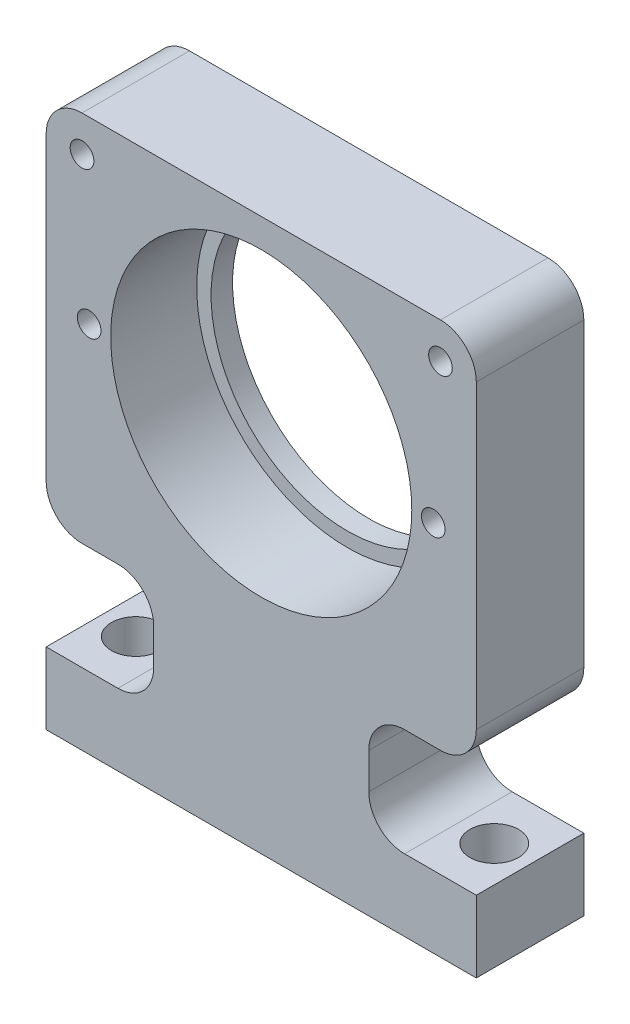
from build123d import *

# Parameters (mm, degrees)
BOSS_EXTRUDE1_DEPTH = 7.5
SKETCH2_R           = 3.4
CUT_EXTRUDE1_DEPTH  = 15
SKETCH4_R           = 19
CUT_EXTRUDE3_DEPTH  = 84.988094394
SKETCH3_R           = 21
CUT_EXTRUDE4_DEPTH  = 12
M4_TAPPED_HOLE2_D   = 3.3
M4_TAPPED_HOLE1_D   = 3.3
FILLET2_R           = 5


with BuildPart() as part:
    # Sketch1 → Boss-Extrude1 (new, symmetric)
    with BuildSketch(Plane.XY):
        Polygon((30, 0), (-30, 0), (-30, 10), (-15, 10), (-15, 25), (-30, 25), (-30, 77), (30, 77), (30, 25), (15, 25), (15, 10), (30, 10), align=None)
    extrude(amount=BOSS_EXTRUDE1_DEPTH, both=True)

    # Sketch2 → Cut-Extrude1 (cut)
    with BuildSketch(Plane.XZ):
        with Locations(Location((-25, 0, 0), (0, 0, 270))):
            Circle(SKETCH2_R)
        with Locations(Location((25, 0, 0), (0, 0, 270))):
            Circle(SKETCH2_R)
    extrude(amount=-CUT_EXTRUDE1_DEPTH, mode=Mode.SUBTRACT)

    # Sketch4 → Cut-Extrude3 (cut, through all)
    with BuildSketch(Plane.XY.offset(7.5)):
        with Locations((0, 52)):
            Circle(SKETCH4_R)
    extrude(amount=-CUT_EXTRUDE3_DEPTH, mode=Mode.SUBTRACT)

    # Sketch3 → Cut-Extrude4 (cut)
    with BuildSketch(Plane.XY.offset(7.5)):
        with Locations((0, 52)):
            Circle(SKETCH3_R)
    extrude(amount=-CUT_EXTRUDE4_DEPTH, mode=Mode.SUBTRACT)

    # M4 Tapped Hole2 (through all)
    with Locations(Plane.XY.offset(7.5)):
        with Locations((24, 52), (-24, 52)):
            Hole(M4_TAPPED_HOLE2_D / 2)

    # M4 Tapped Hole1 (through all)
    with Locations(Plane.XY.offset(7.5)):
        with Locations((-25, 72), (25, 72)):
            Hole(M4_TAPPED_HOLE1_D / 2)

    # Fillet2
    fillet2_edges = [part.edges().sort_by_distance(p)[0] for p in [
        (-30, 25, 0),
        (-30, 77, 0),
        (30, 77, 0),
        (30, 25, 0),
        (15, 25, 0),
        (15, 10, 0),
        (-15, 10, 0),
        (-15, 25, 0),
    ]]
    fillet(fillet2_edges, radius=FILLET2_R)


solid = part.part
